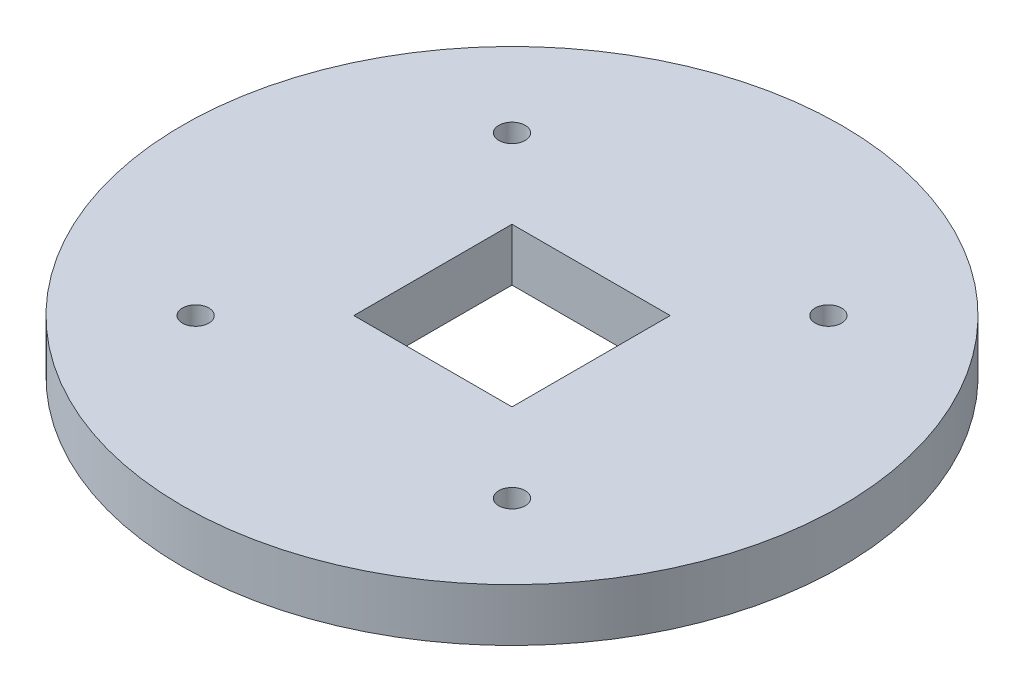
SolidWorks part; units mm, degrees
ref_plane "Front Plane" through (0, 0, 0) normal (0, 0, 1) x (1, 0, 0)
ref_plane "Top Plane" through (0, 0, 0) normal (0, 1, 0) x (1, 0, 0)
ref_plane "Right Plane" through (0, 0, 0) normal (1, 0, 0) x (0, 0, -1)
other "Configuration Table"
sketch "Sketch1" plane through (0, 0, 0) normal (0, 1, 0) x (1, 0, 0)
  line L1 (3, 3) -> (-3, 3)
  line L2 (-3, 3) -> (-3, -3)
  line L3 (-3, -3) -> (3, -3)
  line L4 (3, -3) -> (3, 3)
  circle A0 centre (0, 0) radius 12.5
  circle A2 centre (0, 0) radius 3 construction
  circle A3 centre (-6, 6) radius 0.5
  circle A4 centre (6, 6) radius 0.5
  circle A5 centre (-6, -6) radius 0.5
  circle A6 centre (6, -6) radius 0.5
  dimension "D1" = 25
  dimension "D2" = 6
  dimension "D3" = 1
  dimension "D6" = 1
  dimension "D9" = 1
  dimension "D10" = 1
  dimension "D4" = 3
  dimension "D5" = 3
  dimension "D7" = 3
  dimension "D8" = 3
  dimension "D11" = 3
  dimension "D12" = 3
  dimension "D13" = 3
  dimension "D14" = 3
extrude "Boss-Extrude1" add sketch "Sketch1" along normal blind 2
